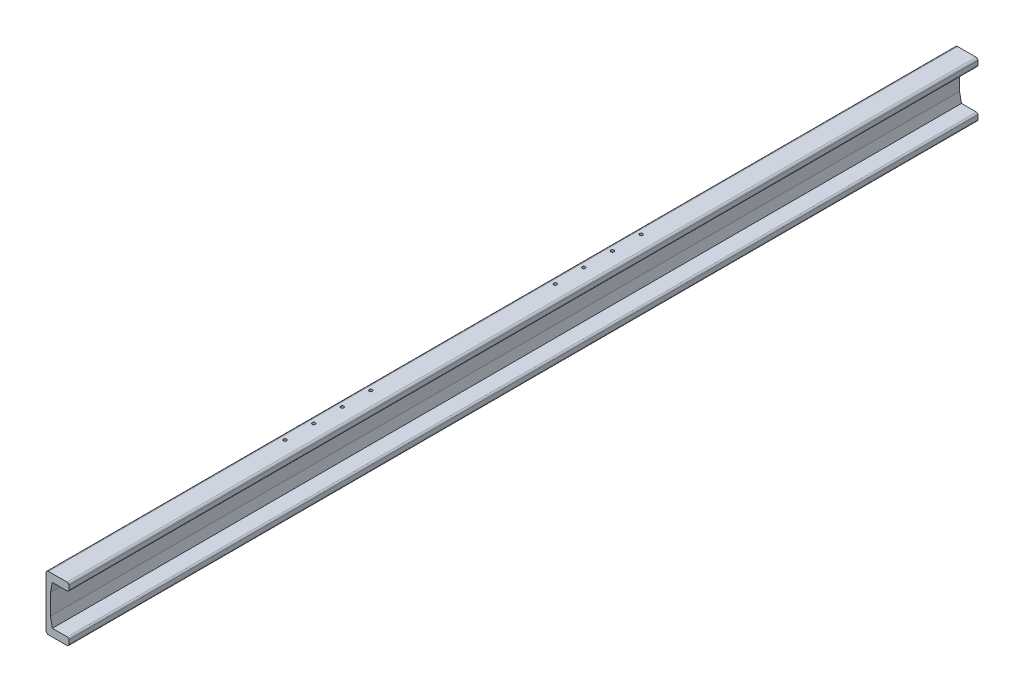
SolidWorks part; units mm, degrees
material "1023 碳钢板 (SS)"
ref_plane "Front Plane" through (0, 0, 0) normal (0, 0, 1) x (1, 0, 0)
ref_plane "Top Plane" through (0, 0, 0) normal (0, 1, 0) x (1, 0, 0)
ref_plane "Right Plane" through (0, 0, 0) normal (1, 0, 0) x (0, 0, -1)
sketch "Sketch1" plane through (0, 0, 0) normal (0, 0, 1) x (1, 0, 0)
  line L0 (-3, 0) -> (-32, 0)
  line L1 (-36, -4) -> (-36, -82.5)
  line L2 (-32, -86.5) -> (-3, -86.5)
  line L3 (0, -83.5) -> (0, -77)
  line L4 (-2.5, -74.5) -> (-26, -74.5)
  line L5 (-29, -59.5) -> (-29, -27)
  line L6 (-26, -12) -> (-2.5, -12)
  line L7 (0, -9.5) -> (0, -3)
  line L8 (-29, -27) -> (-26, -12)
  line L9 (-26, -74.5) -> (-29, -59.5)
  arc A0 (-3, -86.5) -> (0, -83.5) centre (-3, -83.5) ccw
  arc A1 (-3, 0) -> (0, -3) centre (-3, -3) cw
  arc A2 (0, -77) -> (-2.5, -74.5) centre (-2.5, -77) ccw
  arc A3 (-2.5, -12) -> (0, -9.5) centre (-2.5, -9.5) ccw
  arc A4 (-36, -82.5) -> (-32, -86.5) centre (-32, -82.5) ccw
  arc A5 (-32, 0) -> (-36, -4) centre (-32, -4) ccw
  point P15 (0, -86.5)
  point P18 (0, 0)
  point P21 (0, -74.5)
  point P24 (0, -12)
  point P27 (-36, -86.5)
  point P30 (-36, 0)
  dimension "D10" = 3
  dimension "D11" = 2.5
  dimension "D12" = 4
  dimension "D1" = 86.5
  dimension "D2" = 12
  dimension "D3" = 12
  dimension "D4" = 36
  dimension "D5" = 7
  dimension "D6" = 15
  dimension "D7" = 15
  dimension "D8" = 3
  dimension "D9" = 3
extrude "Boss-Extrude1" add sketch "Sketch1" along normal blind 1430 contours L7 A1 L0 A5 L1 A4 L2 A0 L3 A2 L4 L9 L5 L8 L6 A3
sketch "Sketch2" plane through (0, 0, 0) normal (0, 1, 0) x (1, 0, 0)
  line L0 (0, -1430) -> (0, 0) construction
  line L1 (-3, -1430) -> (-32, -1430) construction
  circle A0 centre (-25, -505) radius 2
  circle A2 centre (-25, -550) radius 2
  circle A3 centre (-25, -595) radius 2
  circle A4 centre (-25, -640) radius 2
  circle A5 centre (-25, -1065) radius 2
  circle A6 centre (-25, -1020) radius 2
  circle A7 centre (-25, -975) radius 2
  circle A8 centre (-25, -930) radius 2
  dimension "D2" = 4
  dimension "D6" = 4
  dimension "D3" = 25
  dimension "D5" = 290
  dimension "D7" = 365
  dimension "D1" = 4
  dimension "D4" = 4
hole_wizard "M6 Tapped Hole1" positions "Sketch3" profile "Sketch4" tap size "M6" standard "ISO"
sketch "Sketch3" plane through (0, 0, 0) normal (0, 1, 0) x (1, 0, 0)
  point P0 (-25, -505)
  point P3 (-25, -550)
  point P6 (-25, -595)
  point P9 (-25, -640)
  point P12 (-25, -930)
  point P15 (-25, -975)
  point P18 (-25, -1020)
  point P21 (-25, -1065)
sketch "Sketch4" plane through (-25, 0, 505) normal (1, 0, 0) x (0, 0, 1)
  line L0 (0, 0) -> (0, 16.5022)
  line L1 (0, 16.5022) -> (2.5, 15)
  line L2 (2.5, 15) -> (2.5, 0)
  line L5 (2.5, 0) -> (0, 0)
  line L10 (0, 16.5022) -> (-2.5, 15) construction
  line L11 (0, -6.35) -> (0, 107.95) construction
  dimension "螺纹孔钻头直径" = 5
  dimension "螺纹孔钻头深度" = 15
  dimension "导头角度" = 118
cosmetic thread "Hole thread line 1"
cosmetic thread "Hole thread line 2"
cosmetic thread "Hole thread line 3"
cosmetic thread "Hole thread line 4"
cosmetic thread "Hole thread line 5"
cosmetic thread "Hole thread line 6"
cosmetic thread "Hole thread line 7"
cosmetic thread "Hole thread line 8"
